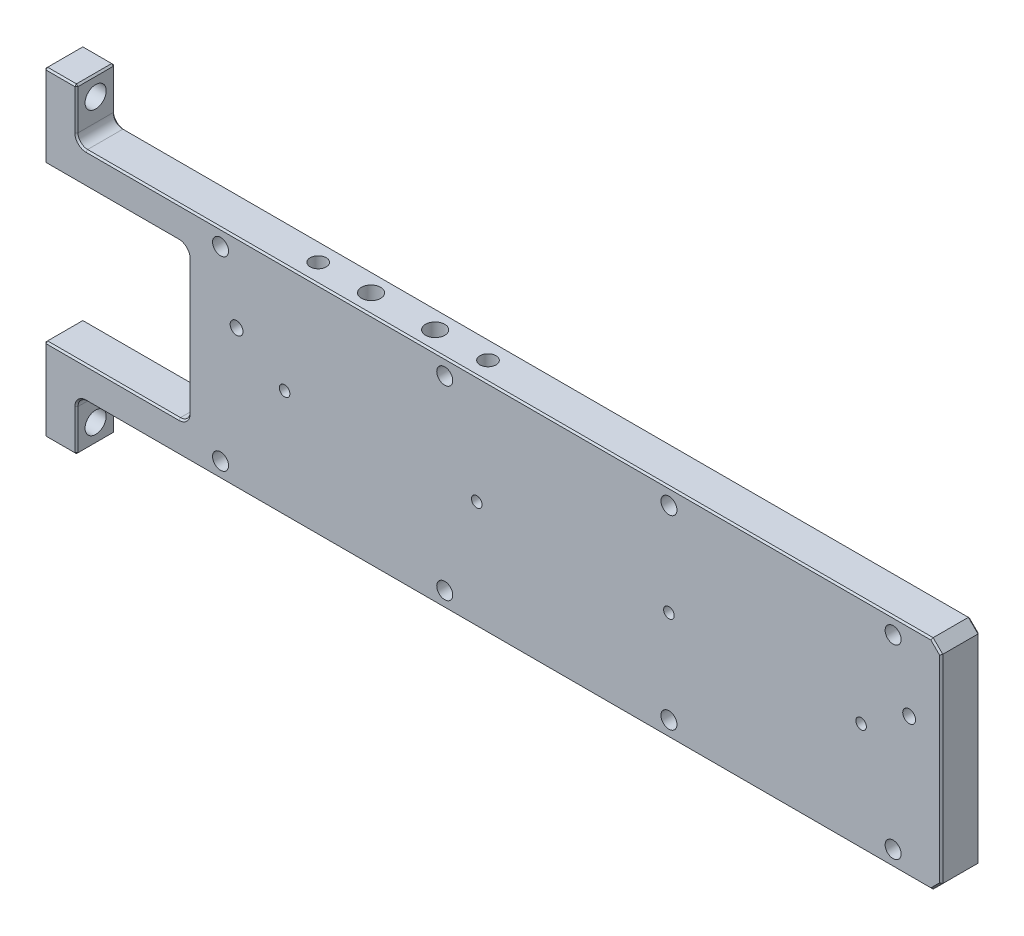
from build123d import *

# Parameters (mm, degrees)
SKETCH_1_W             = 280
SKETCH_1_H             = 68
EXTRUDE_1_DEPTH        = 6
SKETCH_2_W             = 45
SKETCH_2_H             = 48
CUT_EXTRUDE_1_DEPTH    = 25
FILLET_1_R             = 3
SKETCH_3_W             = 12
SKETCH_3_H             = 16
EXTRUDE_2_DEPTH        = 10
FILLET_2_R             = 3
HOLE_WIZARD_M6_1_D     = 6.6
F_6_0MM_1_D            = 6
F_6_0MM_1_DEPTH        = 10
F_6_0MM_1_TIP          = 1.802581857
CHAMFER_1_SIZE         = 3
CHAMFER_2_SIZE         = 0.5
HOLE_WIZARD_M6_3_D     = 5
F_6_0MM_2_D            = 6
F_6_0MM_2_DEPTH        = 6
F_6_0MM_2_TIP          = 1.802581857
HOLE_WIZARD_M6_4_D     = 5
HOLE_WIZARD_M6_4_DEPTH = 15
HOLE_WIZARD_M6_4_TIP   = 1.502151548
HOLE_WIZARD_M4_1_D     = 3.3
F_4_0_MM_1_D           = 4
F_4_0_MM_1_DEPTH       = 5


with BuildPart() as part:
    # 草图1 → 凸台-拉伸1 (new, symmetric)
    with BuildSketch(Plane.XY):
        Rectangle(SKETCH_1_W, SKETCH_1_H)
    extrude(amount=EXTRUDE_1_DEPTH, both=True)

    # 草图2 → 切除-拉伸1 (cut)
    with BuildSketch(Plane(origin=(0, 0, -6), x_dir=(-1, 0, 0), z_dir=(0, 0, -1))):
        with Locations((117.5, 0)):
            Rectangle(SKETCH_2_W, SKETCH_2_H)
    extrude(amount=-CUT_EXTRUDE_1_DEPTH, mode=Mode.SUBTRACT)

    # 圆角1
    fillet_1_edges = [part.edges().sort_by_distance(p)[0] for p in [
        (-95, -24, 0),
        (-95, 24, 0),
    ]]
    fillet(fillet_1_edges, radius=FILLET_1_R)

    # 草图3 → 凸台-拉伸2 (add)
    with BuildSketch(Plane.ZY.offset(140)):
        with Locations((0, -42)):
            Rectangle(SKETCH_3_W, SKETCH_3_H)
        with Locations((0, 42)):
            Rectangle(SKETCH_3_W, SKETCH_3_H)
    extrude(amount=-EXTRUDE_2_DEPTH)

    # 圆角2
    fillet_2_edges = [part.edges().sort_by_distance(p)[0] for p in [
        (-130, -34, 0),
        (-130, 34, 0),
    ]]
    fillet(fillet_2_edges, radius=FILLET_2_R)

    # M6 间隙孔1 (through all)
    with Locations(Plane(origin=(-130, 0, 0), x_dir=(0, 0, -1), z_dir=(1, 0, 0))):
        with Locations((0, -44), (0, 44)):
            Hole(HOLE_WIZARD_M6_1_D / 2)

    # Ø6.0mm 暗销孔1
    with Locations(Plane.ZY.offset(140)):
        with Locations((0, 32.5), (0, -32.5)):
            Hole(F_6_0MM_1_D / 2, depth=F_6_0MM_1_DEPTH)
            with Locations((0, 0, -(F_6_0MM_1_DEPTH + F_6_0MM_1_TIP / 2))):  # 118° drill point
                Cone(0, F_6_0MM_1_D / 2, F_6_0MM_1_TIP, mode=Mode.SUBTRACT)

    # 倒角1
    chamfer_1_edges = [part.edges().sort_by_distance(p)[0] for p in [
        (140, -34, 0),
        (140, 34, 0),
    ]]
    chamfer(chamfer_1_edges, length=CHAMFER_1_SIZE)

    # 倒角2
    chamfer_2_edges = [part.edges().sort_by_distance(p)[0] for p in [
        (-140, 37, 6),
        (5, 34, -6),
        (5, 34, 6),
        (140, 0, -6),
        (138.5, -32.5, -6),
        (138.5, 32.5, -6),
        (140, 0, 6),
        (138.5, -32.5, 6),
        (138.5, 32.5, 6),
        (-140, -37, -6),
        (-140, -37, 6),
        (-119, 24, 6),
        (-140, 24, 0),
        (-140, -24, 0),
        (-119, 24, -6),
        (-119, -24, -6),
        (-119, -24, 6),
        (-95, 0, -6),
        (-95, 0, 6),
        (-95.878679656, -23.121320344, -6),
        (-95.878679656, -23.121320344, 6),
        (-95.878679656, 23.121320344, -6),
        (-95.878679656, 23.121320344, 6),
        (-130, -43.5, 6),
        (-140, 37, -6),
        (-130, -50, 0),
        (-135, -50, 6),
        (-135, -50, -6),
        (-140, -50, 0),
        (-130, 43.5, -6),
        (-130, 50, 0),
        (-135, 50, -6),
        (-135, 50, 6),
        (-140, 50, 0),
        (-130, 43.5, 6),
        (5, -34, 6),
        (5, -34, -6),
        (-130, -43.5, -6),
        (-129.121320344, 34.878679656, 6),
        (-129.121320344, 34.878679656, -6),
        (-129.121320344, -34.878679656, -6),
        (-129.121320344, -34.878679656, 6),
    ]]
    chamfer(chamfer_2_edges, length=CHAMFER_2_SIZE)

    # M6 螺纹孔3 (through all)
    with Locations(Plane(origin=(0, 0, -6), x_dir=(-1, 0, 0), z_dir=(0, 0, -1))):
        with Locations((-125, 29), (-125, -29), (-55, 29), (-55, -29), (15, 29), (15, -29), (85, 29), (85, -29)):
            Hole(HOLE_WIZARD_M6_3_D / 2)

    # Ø6.0mm 暗销孔2
    with Locations(Plane(origin=(0, 34, 0), x_dir=(1, 0, 0), z_dir=(0, 1, 0))):
        with Locations((-24, 0), (-44, 0)):
            Hole(F_6_0MM_2_D / 2, depth=F_6_0MM_2_DEPTH)
            with Locations((0, 0, -(F_6_0MM_2_DEPTH + F_6_0MM_2_TIP / 2))):  # 118° drill point
                Cone(0, F_6_0MM_2_D / 2, F_6_0MM_2_TIP, mode=Mode.SUBTRACT)

    # M6 螺纹孔4
    with Locations(Plane(origin=(0, 34, 0), x_dir=(1, 0, 0), z_dir=(0, 1, 0))):
        with Locations((-7.5, 0), (-60.5, 0)):
            Hole(HOLE_WIZARD_M6_4_D / 2, depth=HOLE_WIZARD_M6_4_DEPTH)
            with Locations((0, 0, -(HOLE_WIZARD_M6_4_DEPTH + HOLE_WIZARD_M6_4_TIP / 2))):  # 118° drill point
                Cone(0, HOLE_WIZARD_M6_4_D / 2, HOLE_WIZARD_M6_4_TIP, mode=Mode.SUBTRACT)

    # M4 螺纹孔1 (through all)
    with Locations(Plane.XY.offset(6)):
        with Locations((115, 0), (55, 0), (-65, 0), (-5, 0)):
            Hole(HOLE_WIZARD_M4_1_D / 2)

    # Ø4.0 mm 暗销孔1
    with Locations(Plane.XY.offset(6)):
        with Locations((-80, 9.5), (130, 9.5)):
            Hole(F_4_0_MM_1_D / 2, depth=F_4_0_MM_1_DEPTH)


solid = part.part
